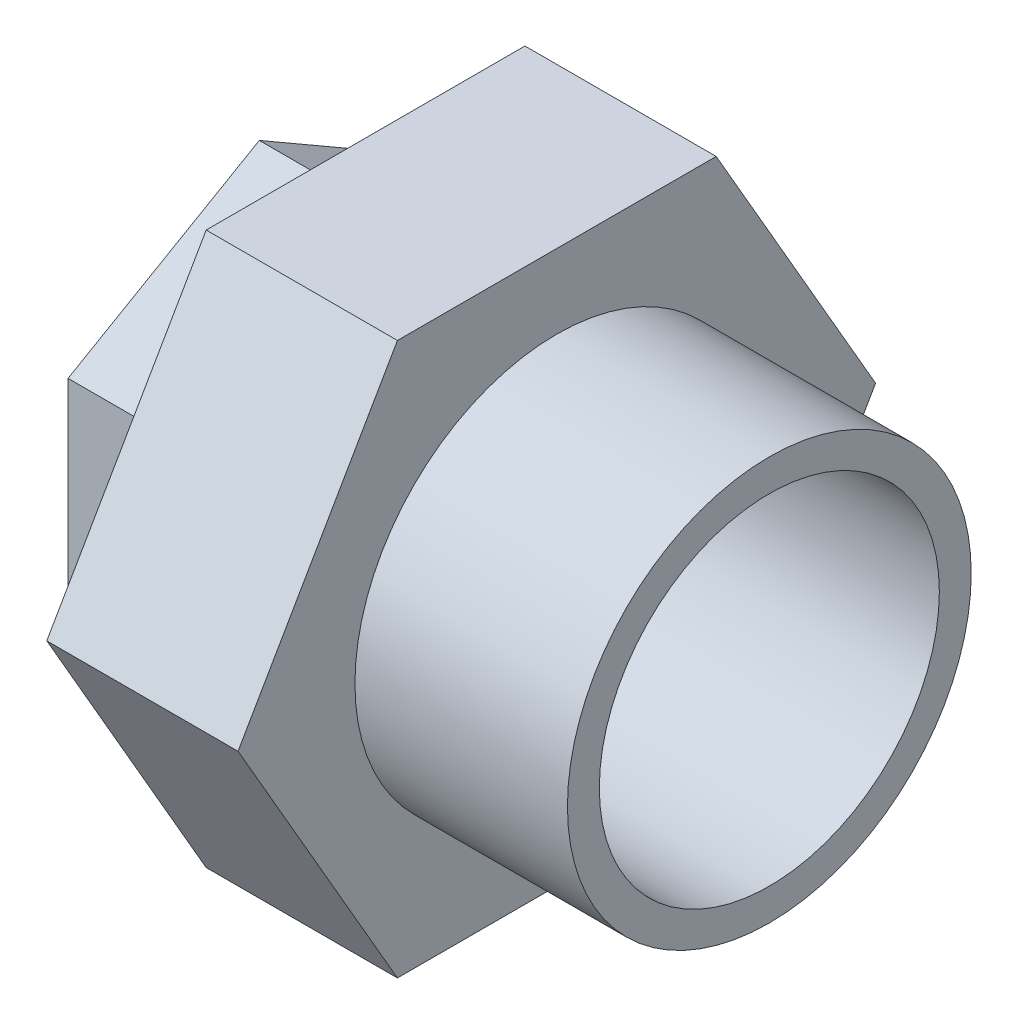
SolidWorks part; units mm, degrees
material "PP 共聚物"
ref_plane "前视基准面" through (0, 0, 0) normal (0, 0, 1) x (1, 0, 0)
ref_plane "上视基准面" through (0, 0, 0) normal (0, 1, 0) x (1, 0, 0)
ref_plane "右视基准面" through (0, 0, 0) normal (1, 0, 0) x (0, 0, -1)
sketch "草图1" plane through (0, 0, 0) normal (1, 0, 0) x (0, 0, -1)
  circle A0 centre (0, 0) radius 16
  dimension "D1" = 32
extrude "拉伸-薄壁1" add sketch "草图1" along normal blind 20 thin
sketch "草图2" plane through (0, 0, 0) normal (-1, 0, 0) x (0, 0, 1)
  line L1 (30, 0) -> (15, 25.9808)
  line L2 (15, 25.9808) -> (-15, 25.9808)
  line L3 (-15, 25.9808) -> (-30, 0)
  line L4 (-30, 0) -> (-15, -25.9808)
  line L5 (-15, -25.9808) -> (15, -25.9808)
  line L6 (15, -25.9808) -> (30, 0)
  circle A0 centre (0, 0) radius 25.9808 construction
  circle A1 centre (0, 0) radius 16
  dimension "D2" = 32
  dimension "D1" = 60
extrude "凸台-拉伸1" add sketch "草图2" along normal blind 18
sketch "草图3" plane through (-18, 0, 0) normal (-1, 0, 0) x (0, 0, 1)
  line L1 (0, 20.7846) -> (-18, 10.3923)
  line L2 (-18, 10.3923) -> (-18, -10.3923)
  line L3 (-18, -10.3923) -> (0, -20.7846)
  line L4 (0, -20.7846) -> (18, -10.3923)
  line L5 (18, -10.3923) -> (18, 10.3923)
  line L6 (18, 10.3923) -> (0, 20.7846)
  circle A0 centre (0, 0) radius 18 construction
  circle A1 centre (0, 0) radius 16.75
  dimension "D1" = 33.5
  dimension "D2" = 36
extrude "凸台-拉伸2" add sketch "草图3" along normal blind 10
